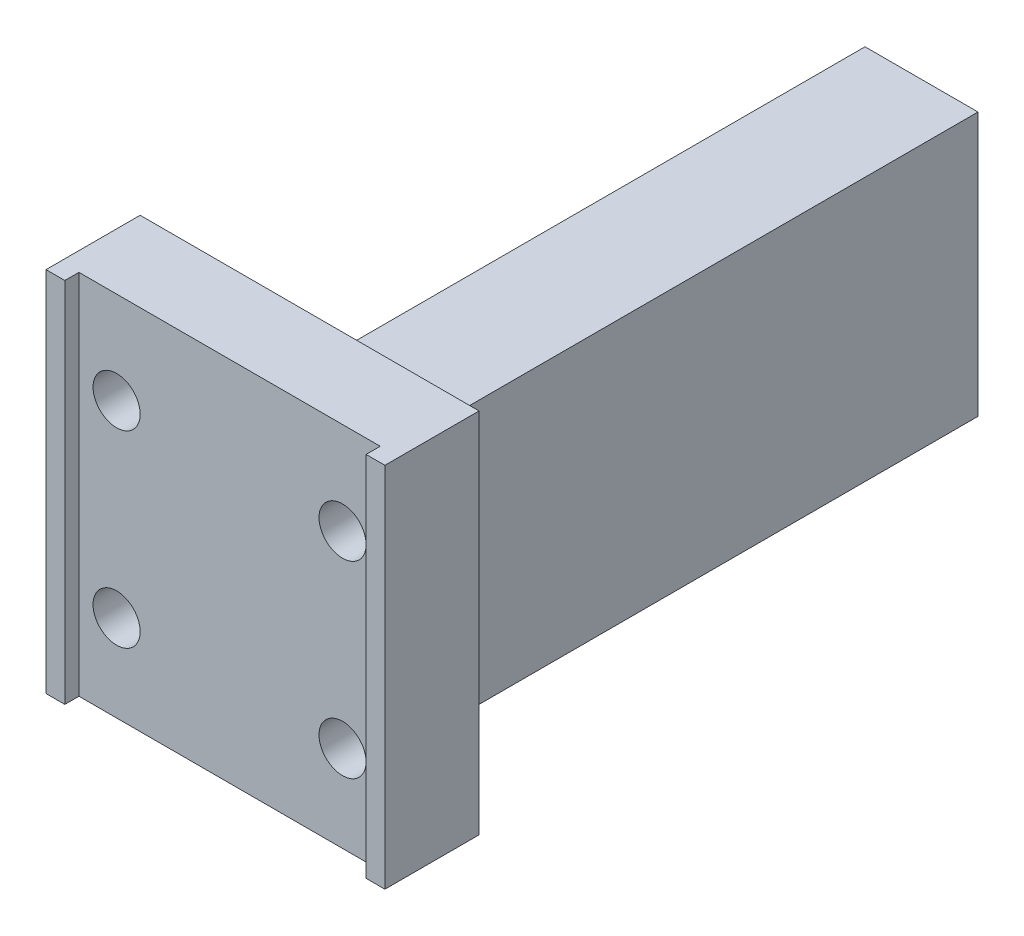
SolidWorks part; units mm, degrees
ref_plane "前视基准面" through (0, 0, 0) normal (0, 0, 1) x (1, 0, 0)
ref_plane "上视基准面" through (0, 0, 0) normal (0, 1, 0) x (1, 0, 0)
ref_plane "右视基准面" through (0, 0, 0) normal (1, 0, 0) x (0, 0, -1)
sketch "草图1" plane through (0, 0, 0) normal (0, 0, 1) x (1, 0, 0)
  line L1 (-18, -19.5) -> (18, -19.5)
  line L2 (-18, -19.5) -> (-18, 19.5)
  line L3 (-18, 19.5) -> (18, 19.5)
  line L4 (18, -19.5) -> (18, 19.5)
  line L5 (-18, -19.5) -> (18, 19.5) construction
  line L6 (-18, 19.5) -> (18, -19.5) construction
  point P0 (0, 0)
  dimension "D1" = 36
  dimension "D2" = 39
extrude "凸台-拉伸1" add sketch "草图1" along normal blind 10
sketch "草图2" plane through (0, 0, 10) normal (0, 0, 1) x (1, 0, 0)
  line L0 (18, 19.5) -> (-18, 19.5) construction
  line L1 (-16, -19.5) -> (16, -19.5)
  line L2 (-16, -19.5) -> (-16, 19.5)
  line L3 (-16, 19.5) -> (16, 19.5)
  line L4 (16, -19.5) -> (16, 19.5)
  line L5 (-16, -19.5) -> (16, 19.5) construction
  line L6 (-16, 19.5) -> (16, -19.5) construction
  point P0 (0, 0)
  dimension "D1" = 32
extrude "切除-拉伸1" cut sketch "草图2" against normal blind 1.5
sketch "草图3" plane through (0, 0, 0) normal (0, 0, -1) x (-1, 0, 0)
  line L1 (-6, -19.5) -> (6, -19.5)
  line L2 (-6, -19.5) -> (-6, 8.5)
  line L3 (-6, 8.5) -> (6, 8.5)
  line L4 (6, -19.5) -> (6, 8.5)
  line L5 (0, -19.5) -> (0, 0) construction
  line L7 (18, -19.5) -> (-18, -19.5) construction
  dimension "D1" = 12
  dimension "D2" = 28
extrude "凸台-拉伸2" add sketch "草图3" along normal blind 65
hole_wizard "Ø5.0 (5) 直径孔1" positions "草图5" profile "草图4" hole size "Ø5.0" standard "GB"
sketch "草图5" plane through (0, 0, 0) normal (0, 0, -1) x (-1, 0, 0)
  circle A0 centre (-12, 9.7) radius 1.621 construction
  circle A1 centre (12, 9.7) radius 1.621 construction
  circle A2 centre (12, -10.3) radius 1.621 construction
  circle A3 centre (-12, -10.3) radius 1.621 construction
  point P1 (-12, 9.7)
  point P5 (12, 9.7)
  point P9 (12, -10.3)
  point P13 (-12, -10.3)
sketch "草图4" plane through (12, 9.7, 0) normal (1, 0, 0) x (0, 1, 0)
  line L0 (0, 0) -> (0, 10)
  line L1 (0, 10) -> (2.5, 10)
  line L2 (2.5, 10) -> (2.5, 0)
  line L5 (2.5, 0) -> (0, 0)
  line L11 (0, -6.35) -> (0, 107.95) construction
  dimension "通孔孔直径" = 5
  dimension "通孔孔深度" = 10
sketch "草图6" plane through (0, 0, -65) normal (0, 0, -1) x (-1, 0, 0)
  line L0 (6, 8.5) -> (-6, 8.5) construction
  line L1 (-90, -19.5) -> (90, -19.5)
  line L2 (-90, -19.5) -> (-90, 8.5)
  line L3 (-90, 8.5) -> (90, 8.5)
  line L4 (90, -19.5) -> (90, 8.5)
  line L5 (-90, -19.5) -> (90, 8.5) construction
  line L6 (-90, 8.5) -> (90, -19.5) construction
  line L7 (-6, -19.5) -> (6, -19.5) construction
  point P0 (0, -5.5)
  dimension "D1" = 180
extrude "凸台-拉伸3" [suppressed] add sketch "草图6" along normal blind 12
sketch "草图7" [suppressed] plane through (0, 0, -30) normal (0, 0, 1) x (1, 0, 0)
  line L0 (15, 20.5) -> (80, 20.5) construction
  line L1 (15, 23.5) -> (80, 23.5)
  line L2 (15, 17.5) -> (80, 17.5)
  line L3 (6, 27.5) -> (90, 27.5) construction
  line L4 (90, 27.5) -> (90, -0.5) construction
  line L5 (0, 0) -> (0, -27.5) construction
  line L6 (-16, -27.5) -> (16, -27.5) construction
  line L7 (-15, 20.5) -> (-80, 20.5) construction
  line L8 (-15, 23.5) -> (-80, 23.5)
  line L9 (-15, 17.5) -> (-80, 17.5)
  line L10 (90, 13.5) -> (-90, 13.5) construction
  line L11 (-90, -0.5) -> (-90, 27.5) construction
  line L12 (-15, 6.5) -> (-80, 6.5) construction
  line L13 (-15, 3.5) -> (-80, 3.5)
  line L14 (-15, 9.5) -> (-80, 9.5)
  line L15 (15, 6.5) -> (80, 6.5) construction
  line L16 (15, 3.5) -> (80, 3.5)
  line L17 (15, 9.5) -> (80, 9.5)
  arc A0 (15, 23.5) -> (15, 17.5) centre (15, 20.5) ccw
  arc A1 (80, 17.5) -> (80, 23.5) centre (80, 20.5) ccw
  arc A2 (-15, 23.5) -> (-15, 17.5) centre (-15, 20.5) cw
  arc A3 (-80, 17.5) -> (-80, 23.5) centre (-80, 20.5) cw
  arc A4 (-15, 3.5) -> (-15, 9.5) centre (-15, 6.5) ccw
  arc A5 (-80, 9.5) -> (-80, 3.5) centre (-80, 6.5) ccw
  arc A6 (15, 3.5) -> (15, 9.5) centre (15, 6.5) cw
  arc A7 (80, 9.5) -> (80, 3.5) centre (80, 6.5) cw
  point P2 (47.5, 20.5)
  point P18 (-47.5, 20.5)
  point P29 (-47.5, 6.5)
  point P36 (47.5, 6.5)
  dimension "D1" = 3
  dimension "D2" = 4
  dimension "D3" = 65
  dimension "D4" = 10
extrude "切除-拉伸2" [suppressed] cut sketch "草图7" against normal up to next
